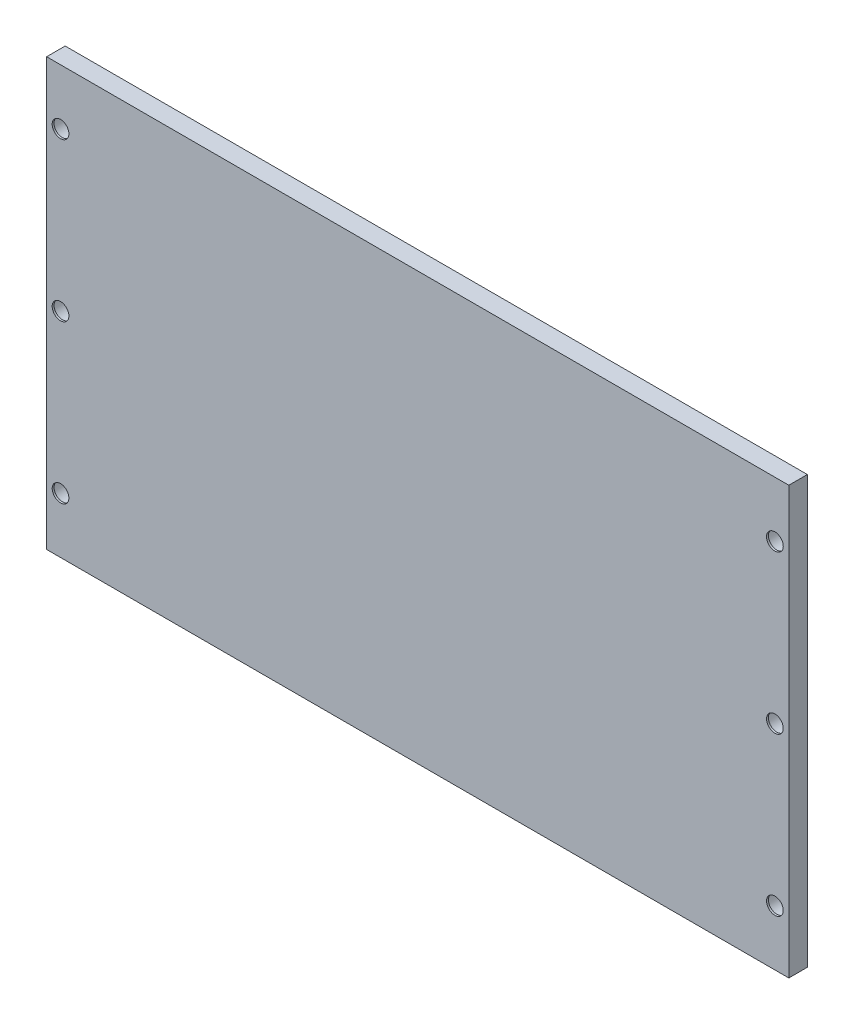
SolidWorks part; units mm, degrees
ref_plane "Front Plane" through (0, 0, 0) normal (0, 0, 1) x (1, 0, 0)
ref_plane "Top Plane" through (0, 0, 0) normal (0, 1, 0) x (1, 0, 0)
ref_plane "Right Plane" through (0, 0, 0) normal (1, 0, 0) x (0, 0, -1)
sketch "Sketch1" plane through (0, 0, 0) normal (0, 0, 1) x (1, 0, 0)
  line L2 (200, -115) -> (-200, -115)
  line L3 (200, -115) -> (200, 115)
  line L4 (200, 115) -> (-200, 115)
  line L5 (-200, -115) -> (-200, 115)
  line L6 (200, -115) -> (-200, 115) construction
  line L7 (200, 115) -> (-200, -115) construction
  point P2 (0, 0)
  dimension "D1" = 400
  dimension "D2" = 230
extrude "Boss-Extrude1" add sketch "Sketch1" along normal blind 10
sketch "Sketch2" plane through (0, 0, 0) normal (0, 0, -1) x (-1, 0, 0)
  circle A0 centre (192.5, -85) radius 4.5
  circle A1 centre (192.5, 0) radius 4.5
  circle A2 centre (192.5, 85) radius 4.5
  dimension "D1" = 9
  dimension "D2" = 9
  dimension "D3" = 9
extrude "Cut-Extrude1" cut sketch "Sketch2" against normal blind 25
sketch "Sketch3" plane through (0, 0, 0) normal (0, 0, -1) x (-1, 0, 0)
  circle A0 centre (192.5, -85) radius 6.5
  circle A1 centre (192.5, 0) radius 6.5
  circle A2 centre (192.5, 85) radius 6.5
  dimension "D1" = 13
  dimension "D2" = 13
  dimension "D3" = 13
extrude "Cut-Extrude2" cut sketch "Sketch3" against normal blind 9
mirror "Mirror1" about plane through (0, 0, 0) normal (1, 0, 0) of "Cut-Extrude2", "Cut-Extrude1"
